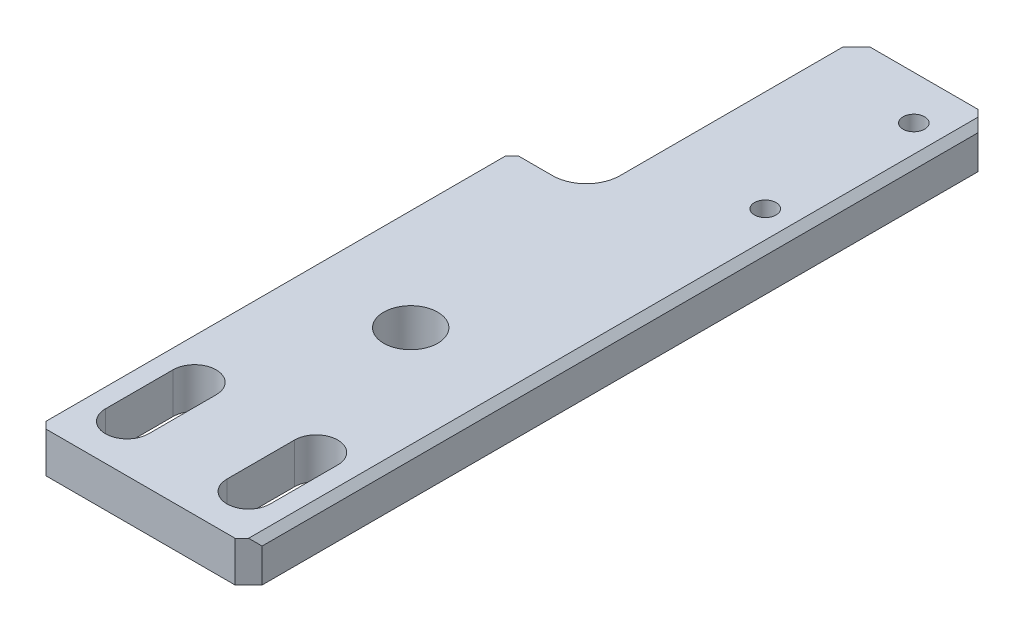
SolidWorks part; units mm, degrees
ref_plane "Front Plane" through (0, 0, 0) normal (0, 0, 1) x (1, 0, 0)
ref_plane "Top Plane" through (0, 0, 0) normal (0, 1, 0) x (1, 0, 0)
ref_plane "Right Plane" through (0, 0, 0) normal (1, 0, 0) x (0, 0, -1)
sketch "Sketch1" plane through (0, 0, 0) normal (0, 1, 0) x (1, 0, 0)
  line L1 (0, 0) -> (16, 0)
  line L2 (0, 0) -> (0, -55)
  line L3 (0, -55) -> (16, -55)
  line L4 (16, 0) -> (16, -55)
  dimension "D1" = 16
  dimension "D2" = 55
extrude "Boss-Extrude1" add sketch "Sketch1" along normal blind 3
sketch "Sketch4" plane through (0, 0, 0) normal (0, -1, 0) x (1, 0, 0)
  line L0 (8, 60) -> (8, -49940) construction
  line L1 (0, 55) -> (16, 55) construction
  line L2 (3.5, 51.5) -> (3.5, 46.5) construction
  line L3 (5.1, 51.5) -> (5.1, 46.5)
  line L4 (1.9, 51.5) -> (1.9, 46.5)
  line L5 (12.5, 51.5) -> (12.5, 46.5) construction
  line L6 (10.9, 51.5) -> (10.9, 46.5)
  line L7 (14.1, 51.5) -> (14.1, 46.5)
  arc A0 (5.1, 51.5) -> (1.9, 51.5) centre (3.5, 51.5) ccw
  arc A1 (1.9, 46.5) -> (5.1, 46.5) centre (3.5, 46.5) ccw
  arc A2 (10.9, 51.5) -> (14.1, 51.5) centre (12.5, 51.5) cw
  arc A3 (14.1, 46.5) -> (10.9, 46.5) centre (12.5, 46.5) cw
  point P4 (8, 55)
  point P7 (3.5, 49)
  point P14 (12.5, 49)
  dimension "D1" = 3.2
  dimension "D2" = 9
  dimension "D3" = 5
  dimension "D4" = 6
extrude "Cut-Extrude2" cut sketch "Sketch4" against normal blind 10
sketch "Sketch5" plane through (0, 3, 0) normal (0, 1, 0) x (1, 0, 0)
  line L1 (0, 0) -> (6, 0)
  line L2 (0, 0) -> (0, -20)
  line L3 (0, -20) -> (6, -20)
  line L4 (6, 0) -> (6, -20)
  dimension "D1" = 20
  dimension "D2" = 6
extrude "Cut-Extrude3" cut sketch "Sketch5" against normal blind 10
fillet "Fillet1" radius 2.5 1 edges at (6, 1.5, 20)
chamfer "Chamfer1" distance 1 angle 45 5 edges at (6, 1.5, 0) (16, 1.5, 0) (16, 1.5, 55) (0, 1.5, 55) (0, 1.5, 20)
chamfer "Chamfer2" distance 0.5 angle 45 2 edges at (16, 3, 27.5) (0, 3, 37.5)
hole_wizard "M2 Tapped Hole1" positions "Sketch7" profile "Sketch6" tap size "M2" standard "Gb"
sketch "Sketch7" plane through (0, 3, 0) normal (0, 1, 0) x (1, 0, 0)
  line L0 (13.5, -3.25) -> (13.5, -14.25) construction
  line L2 (16, -1) -> (16, -54) construction
  line L3 (15, 0) -> (7, 0) construction
  point P0 (13.5, -3.25)
  point P3 (13.5, -14.25)
  dimension "D1" = 2.5
  dimension "D2" = 11
  dimension "D3" = 3.25
sketch "Sketch6" plane through (13.5, 3, 3.25) normal (1, 0, 0) x (0, 0, 1)
  line L0 (0, 0) -> (0, 5.6807)
  line L1 (0, 5.6807) -> (0.8, 5.2)
  line L2 (0.8, 5.2) -> (0.8, 0)
  line L5 (0.8, 0) -> (0, 0)
  line L10 (0, 5.6807) -> (-0.8, 5.2) construction
  line L11 (0, -6.35) -> (0, 107.95) construction
  dimension "螺纹孔钻头直径" = 1.6
  dimension "螺纹孔钻头深度" = 5.2
  dimension "导头角度" = 118
cosmetic thread "Hole thread 1" parameters "D1"=3, "D2"=2
cosmetic thread "Hole thread 2" parameters "D1"=3, "D2"=2
hole_wizard "Ø4.0 (4) Diameter Hole1" positions "Sketch9" profile "Sketch8" hole size "Ø4.0" standard "Gb"
sketch "Sketch9" plane through (0, 0, 0) normal (0, -1, 0) x (-1, 0, 0)
  line L0 (-1, -55) -> (-15, -55) construction
  line L1 (-8, -55) -> (-8, -24.6588) construction
  point P0 (-8, -35)
  dimension "D1" = 20
sketch "Sketch8" plane through (8, 0, 35) normal (1, 0, 0) x (0, 0, -1)
  line L0 (0, 0) -> (0, 5.2017)
  line L1 (0, 5.2017) -> (2, 4)
  line L2 (2, 4) -> (2, 0)
  line L5 (2, 0) -> (0, 0)
  line L10 (0, 5.2017) -> (-2, 4) construction
  line L11 (0, -6.35) -> (0, 107.95) construction
  dimension "孔直径" = 4
  dimension "孔深度" = 4
  dimension "导头角度" = 118
